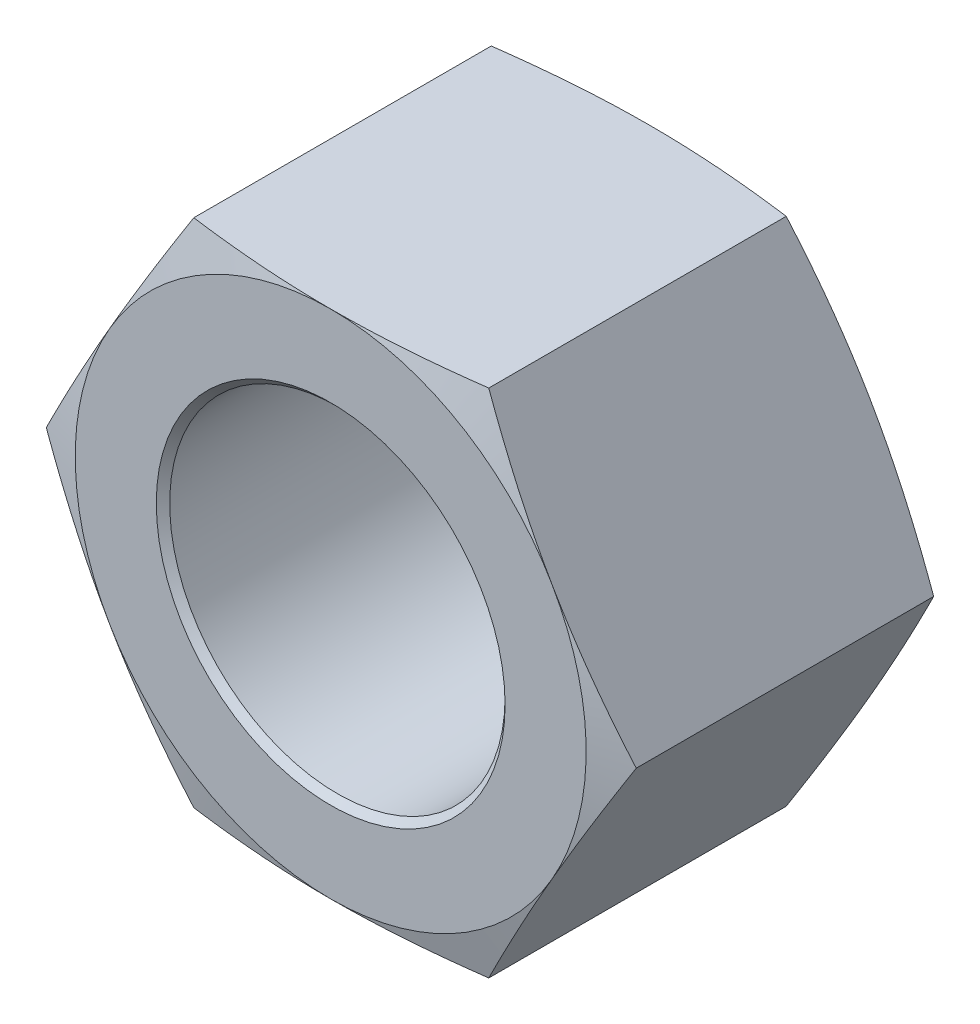
SolidWorks part; units mm, degrees
ref_plane "Plane1" through (0, 0, 0) normal (0, 0, 1) x (1, 0, 0)
ref_plane "Plane2" through (0, 0, 0) normal (0, 1, 0) x (1, 0, 0)
ref_plane "Plane3" through (0, 0, 0) normal (1, 0, 0) x (0, 0, -1)
sketch "Dimension Sketch" plane through (0, 0, 0) normal (0, 0, 1) x (1, 0, 0)
  line L0 (0, 0) -> (24.1005, 0)
  point P3 (10, 0)
  point P4 (1.5, 0)
  point P5 (17.59, 0)
  point P6 (9.5, 0)
  point P7 (6.4, 0)
  point P8 (16, 0)
sketch "Sketch1" plane through (0, 0, 0) normal (0, 0, 1) x (1, 0, 0)
  line L0 (-26.8088, 0) -> (37.1748, 0) construction
  line L1 (0, 25.0215) -> (0, -25.0215) construction
  line L3 (4.3975, 7.6167) -> (-4.3975, 7.6167)
  line L4 (-4.3975, 7.6167) -> (-8.795, 0)
  line L5 (-8.795, 0) -> (-4.3975, -7.6167)
  line L6 (-4.3975, -7.6167) -> (4.3975, -7.6167)
  line L7 (4.3975, -7.6167) -> (8.795, 0)
  line L8 (8.795, 0) -> (4.3975, 7.6167)
  circle A0 centre (0, 0) radius 7.6167 construction
  circle A1 centre (0, 0) radius 5
extrude "Boss-Extrude" add sketch "Sketch1" along normal blind 9.5
cosmetic thread "Cosmetic Thread1" parameters "D2"=10.5
sketch "Sketch2" plane through (0, 0, 0) normal (0, 0, -1) x (-1, 0, 0)
  line L0 (-4.3975, 7.6167) -> (4.3975, 7.6167) construction
  circle A0 centre (0, 0) radius 7.6167
  circle A1 centre (0, 0) radius 5 construction
extrude "Cut-Extrude1" cut sketch "Sketch2" against normal blind 38 draft 75 flip side to cut
sketch "Sketch3" plane through (0, 0, 9.5) normal (0, 0, 1) x (1, 0, 0)
  line L0 (8.795, 0) -> (4.3975, 7.6167) construction
  circle A0 centre (0, 0) radius 7.6167
extrude "Cut-Extrude2" cut sketch "Sketch3" against normal blind 38 draft 75 flip side to cut
chamfer "Chamfer1" distance 0.2 angle 45 2 edges at (5, 0, 0) (5, 0, 9.5)
equation "\"e@Sketch1\" = \"e@Dimension Sketch\""
equation "\"D@Sketch1\" = \"D@Dimension Sketch\""
equation "\"m@Boss-Extrude\" = \"m@Dimension Sketch\""
equation "\"D2@Cosmetic Thread1\" = 1.05 * \"D@Dimension Sketch\""
